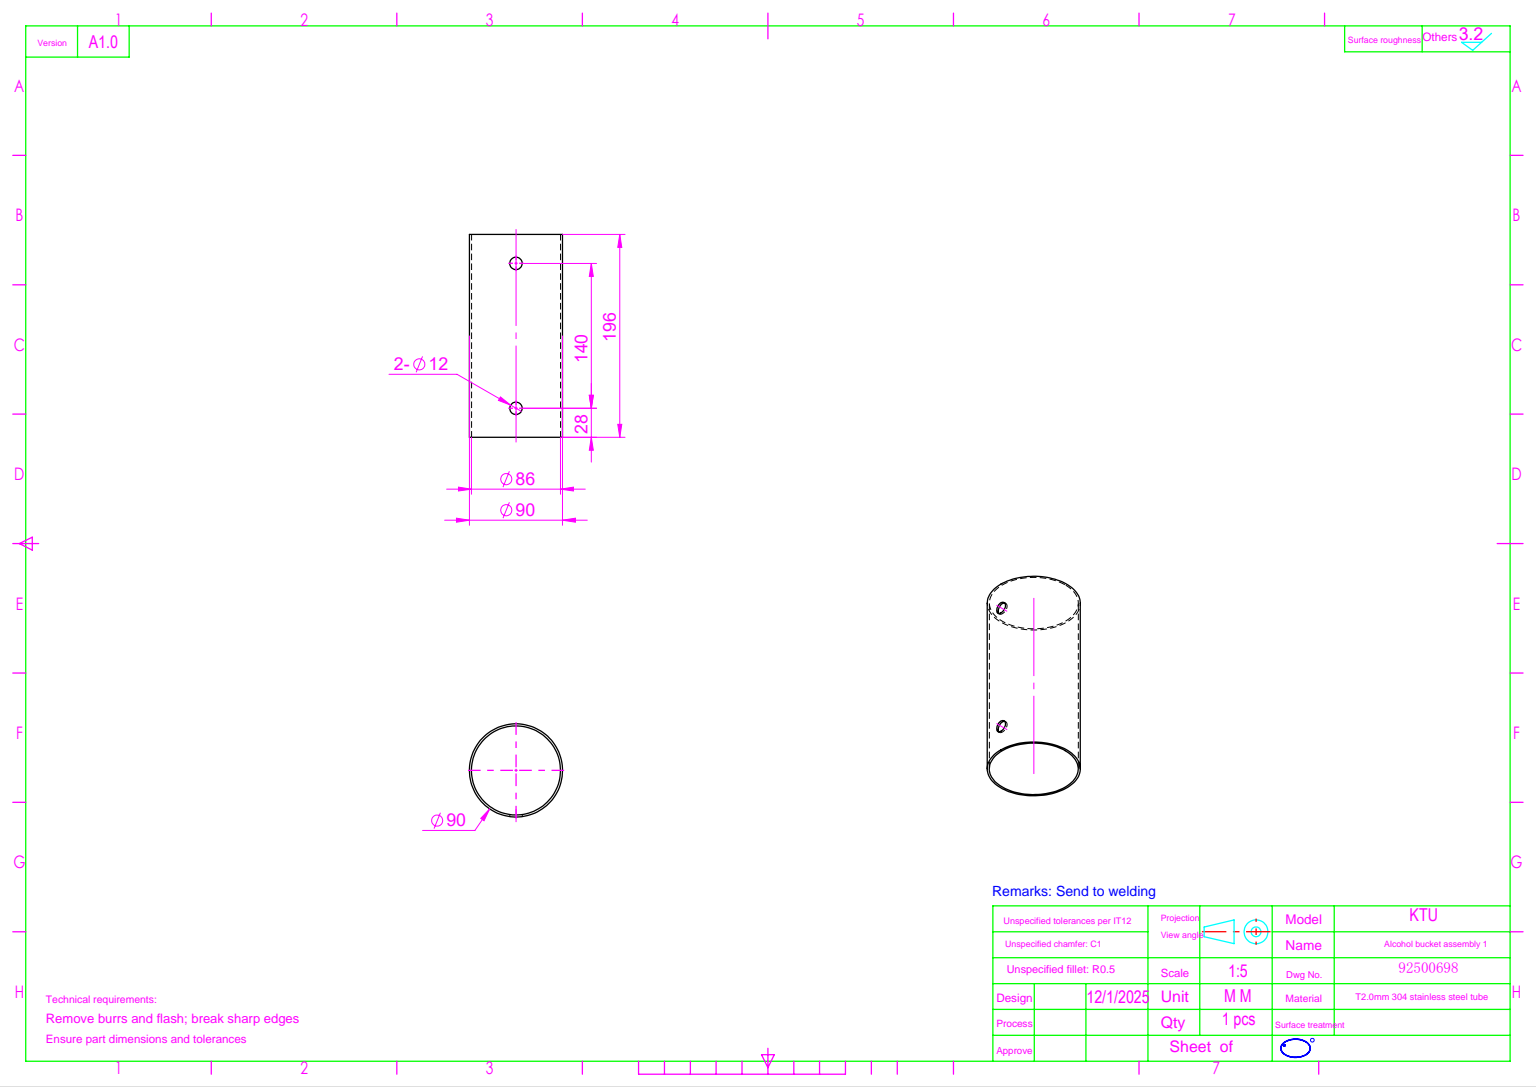
from build123d import *

# Parameters (mm, degrees)
SKETCH_2_R          = 45
SKETCH_2_R_2        = 43
EXTRUDE_1_DEPTH     = 98
SKETCH_3_R          = 6
CUT_EXTRUDE_2_DEPTH = 117.850331621


with BuildPart() as part:
    # 草图2 → 拉伸-薄壁1 (new, symmetric)
    with BuildSketch(Plane(origin=(0, 0, 0), x_dir=(1, 0, 0), z_dir=(0, 1, 0))):
        Circle(SKETCH_2_R)
        Circle(SKETCH_2_R_2, mode=Mode.SUBTRACT)
    extrude(amount=EXTRUDE_1_DEPTH, both=True)

    # 草图3 → 切除-拉伸2 (cut, through all)
    with BuildSketch(Plane.XY):
        with Locations(Location((0, 70, 0), (0, 0, 180))):
            Circle(SKETCH_3_R)
        with Locations(Location((0, -70, 0), (0, 0, 180))):
            Circle(SKETCH_3_R)
    extrude(amount=CUT_EXTRUDE_2_DEPTH, mode=Mode.SUBTRACT)


solid = part.part
